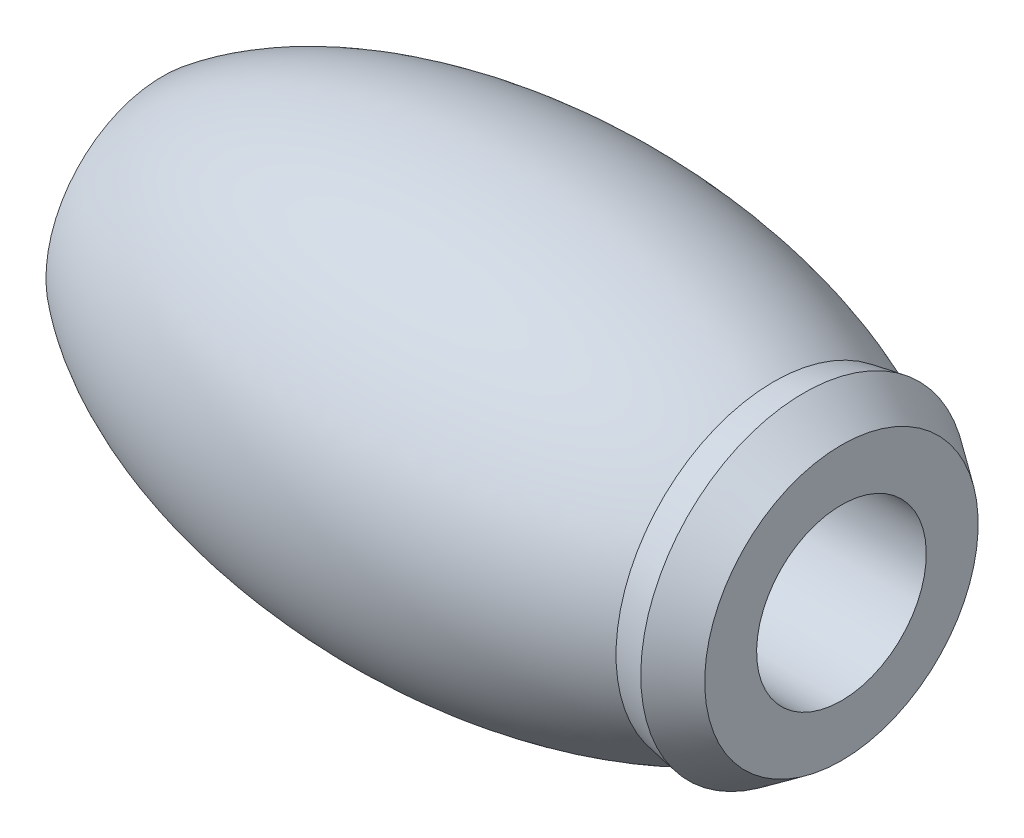
SolidWorks part; units mm, degrees
ref_plane "Front Plane" through (0, 0, 0) normal (0, 0, 1) x (1, 0, 0)
ref_plane "Top Plane" through (0, 0, 0) normal (0, 1, 0) x (1, 0, 0)
ref_plane "Right Plane" through (0, 0, 0) normal (1, 0, 0) x (0, 0, -1)
sketch "Sketch1" plane through (0, 0, 0) normal (0, 0, 1) x (1, 0, 0)
  line L0 (-40, 0) -> (40, 0)
  line L1 (40, 25) -> (-40, 25)
  line L2 (40, 25) -> (40, -25)
  line L3 (40, -25) -> (-40, -25)
  line L4 (-40, 25) -> (-40, -25)
  line L5 (40, 25) -> (-40, -25) construction
  line L6 (40, -25) -> (-40, 25) construction
  line L7 (42.7528, 0) -> (77.0773, 0) construction
  line L8 (-40, 10) -> (40, 10)
  line L9 (-40, -10) -> (40, -10)
  ellipse E0 centre (0, 0) end of major axis (47.9073, 0) minor radius 25 (-40, -13.7583) -> (40, -13.7583) ccw
  ellipse E1 centre (0, 0) end of major axis (47.9073, 0) minor radius 25 (40, 13.7583) -> (-40, 13.7583) ccw
  ellipse E2 centre (0, 0) end of major axis (44.9073, 0) minor radius 22 (-40, -10) -> (40, -10) ccw
  ellipse E3 centre (0, 0) end of major axis (44.9073, 0) minor radius 22 (40, 10) -> (-40, 10) ccw
  point P0 (0, 0)
  dimension "D1" = 80
  dimension "D2" = 50
  dimension "D3" = 3
  dimension "D4" = 3
  dimension "D5" = 10
revolve "Revolve2" add sketch "Sketch1" angle 360 about L7
sketch "Sketch2" plane through (40, 0, 0) normal (1, 0, 0) x (0, 0, -1)
  circle A0 centre (0, 0) radius 13.7583
  circle A1 centre (0, 0) radius 20
  circle A2 centre (0, 0) radius 13.7583 construction
  dimension "D1" = 40
extrude "Boss-Extrude2" add sketch "Sketch2" against normal up to next (9.8644 mm away) draft 10
chamfer "Chamfer2" distance 4.5 angle 45 1 edges at (40, 20, 0)
